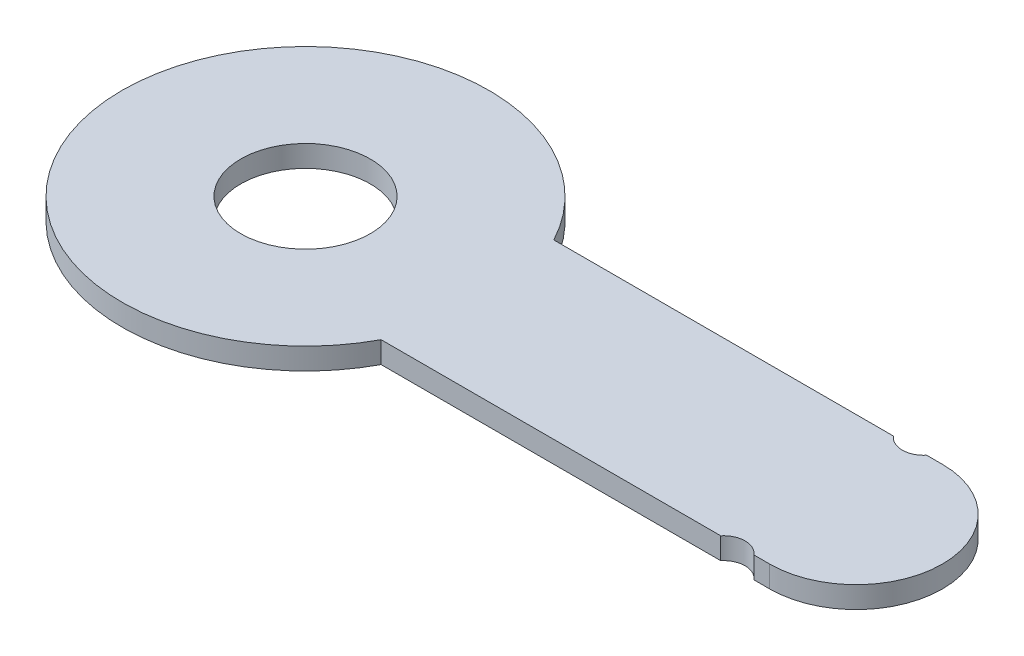
SolidWorks part; units mm, degrees
ref_plane "Front Plane" through (0, 0, 0) normal (0, 0, 1) x (1, 0, 0)
ref_plane "Top Plane" through (0, 0, 0) normal (0, 1, 0) x (1, 0, 0)
ref_plane "Right Plane" through (0, 0, 0) normal (1, 0, 0) x (0, 0, -1)
sketch "Sketch1" plane through (0, 0, 0) normal (0, 1, 0) x (1, 0, 0)
  line L0 (0, 0) -> (12.75, 0) construction
  line L1 (12.75, 2) -> (3.75, 2)
  line L2 (12.75, -2) -> (3.75, -2)
  arc A0 (3.75, 2) -> (3.75, -2) centre (0, 0) ccw
  arc A1 (12.75, -2) -> (12.75, 2) centre (12.75, 0) ccw
  circle A2 centre (0, 0) radius 1.5
  dimension "D2" = 19
  dimension "D3" = 8.5
  dimension "D4" = 3
  dimension "D1" = 4
extrude "Boss-Extrude1" add sketch "Sketch1" along normal blind 0.5
sketch "Sketch2" plane through (0, 0.5, 0) normal (0, 1, 0) x (1, 0, 0)
  circle A0 centre (12, 2.32) radius 0.5
  circle A1 centre (12, -2.32) radius 0.5
  circle A2 centre (0, 0) radius 1.5 construction
  dimension "D1" = 1
  dimension "D2" = 13.5
  dimension "D3" = 3.64
  dimension "D4" = 1.82
extrude "Cut-Extrude1" cut sketch "Sketch2" against normal through all
